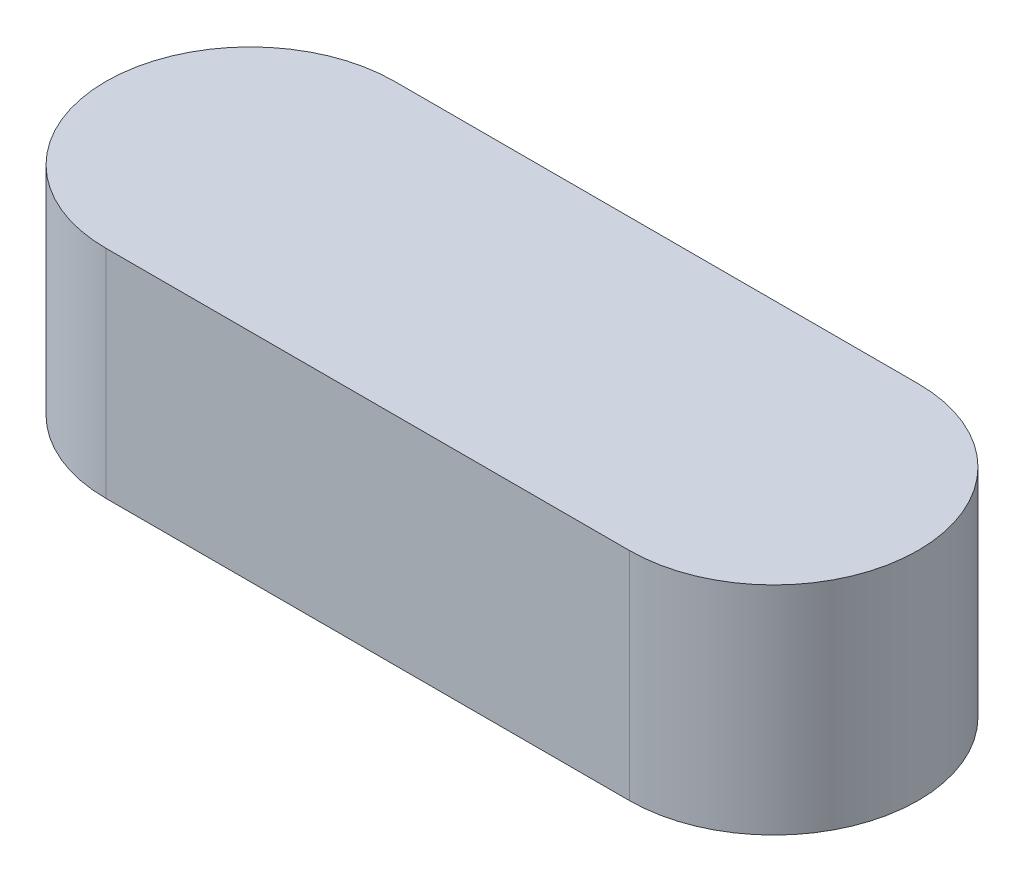
SolidWorks part; units mm, degrees
ref_plane "Front" through (0, 0, 0) normal (0, 0, 1) x (1, 0, 0)
ref_plane "Top" through (0, 0, 0) normal (0, 1, 0) x (1, 0, 0)
ref_plane "Right" through (0, 0, 0) normal (1, 0, 0) x (0, 0, -1)
sketch "Sketch1" plane through (0, 0, 0) normal (0, 1, 0) x (1, 0, 0)
  line L0 (0, 0) -> (29, 0) construction
  line L1 (0, 8) -> (29, 8)
  line L2 (0, -8) -> (29, -8)
  arc A0 (0, 8) -> (0, -8) centre (0, 0) ccw
  arc A1 (29, -8) -> (29, 8) centre (29, 0) ccw
  point P3 (14.5, 0)
  dimension "D2" = 8
  dimension "D1" = 29
extrude "Boss-Extrude1" add sketch "Sketch1" along normal blind 12
